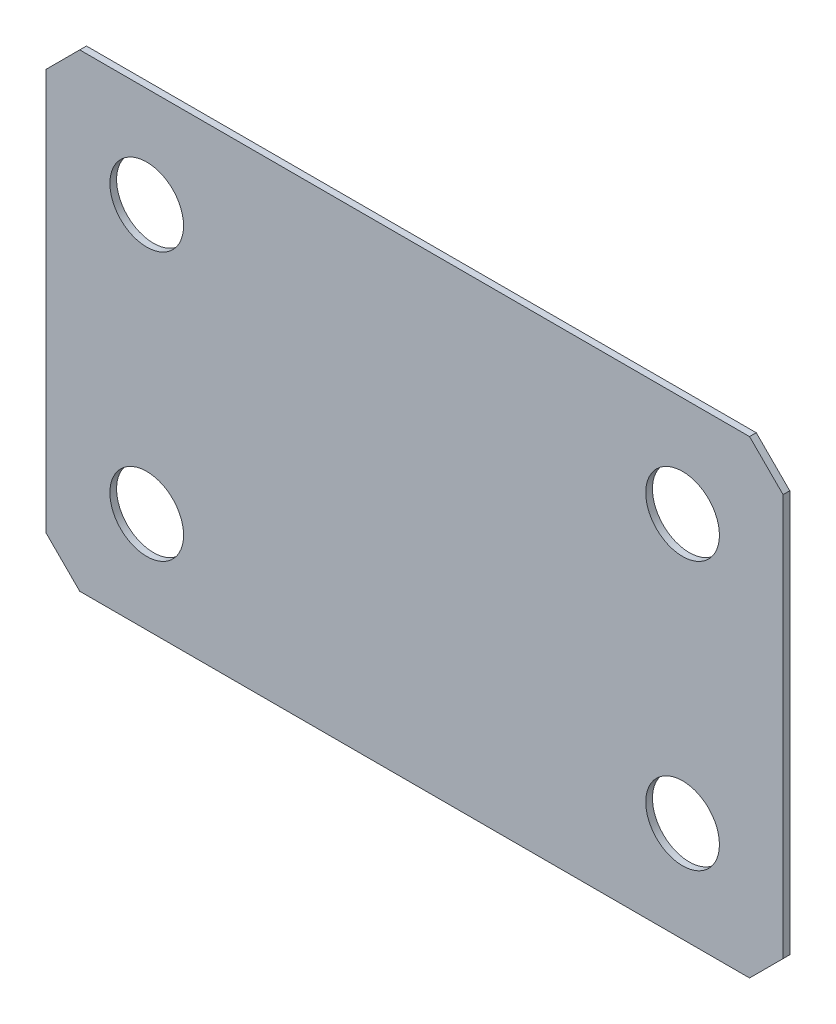
from build123d import *

# Parameters (mm, degrees)
SKETCH1_W           = 110
SKETCH1_H           = 70
BOSS_EXTRUDE1_DEPTH = 1
SKETCH2_R           = 5.5
CUT_EXTRUDE1_DEPTH  = 1
CHAMFER1_SIZE       = 5


with BuildPart() as part:
    # Sketch1 → Boss-Extrude1 (new body)
    with BuildSketch(Plane.XY):
        Rectangle(SKETCH1_W, SKETCH1_H)
    extrude(amount=BOSS_EXTRUDE1_DEPTH)

    # Sketch2 → Cut-Extrude1 (cut)
    with BuildSketch(Plane.XY.offset(1)):
        with Locations((-40, 20)):
            Circle(SKETCH2_R)
        with Locations((40, 20)):
            Circle(SKETCH2_R)
        with Locations((-40, -20)):
            Circle(SKETCH2_R)
        with Locations((40, -20)):
            Circle(SKETCH2_R)
    extrude(amount=-CUT_EXTRUDE1_DEPTH, mode=Mode.SUBTRACT)

    # Chamfer1
    chamfer1_edges = [part.edges().sort_by_distance(p)[0] for p in [
        (-55, 35, 0.5),
        (55, 35, 0.5),
        (55, -35, 0.5),
        (-55, -35, 0.5),
    ]]
    chamfer(chamfer1_edges, length=CHAMFER1_SIZE)


solid = part.part
